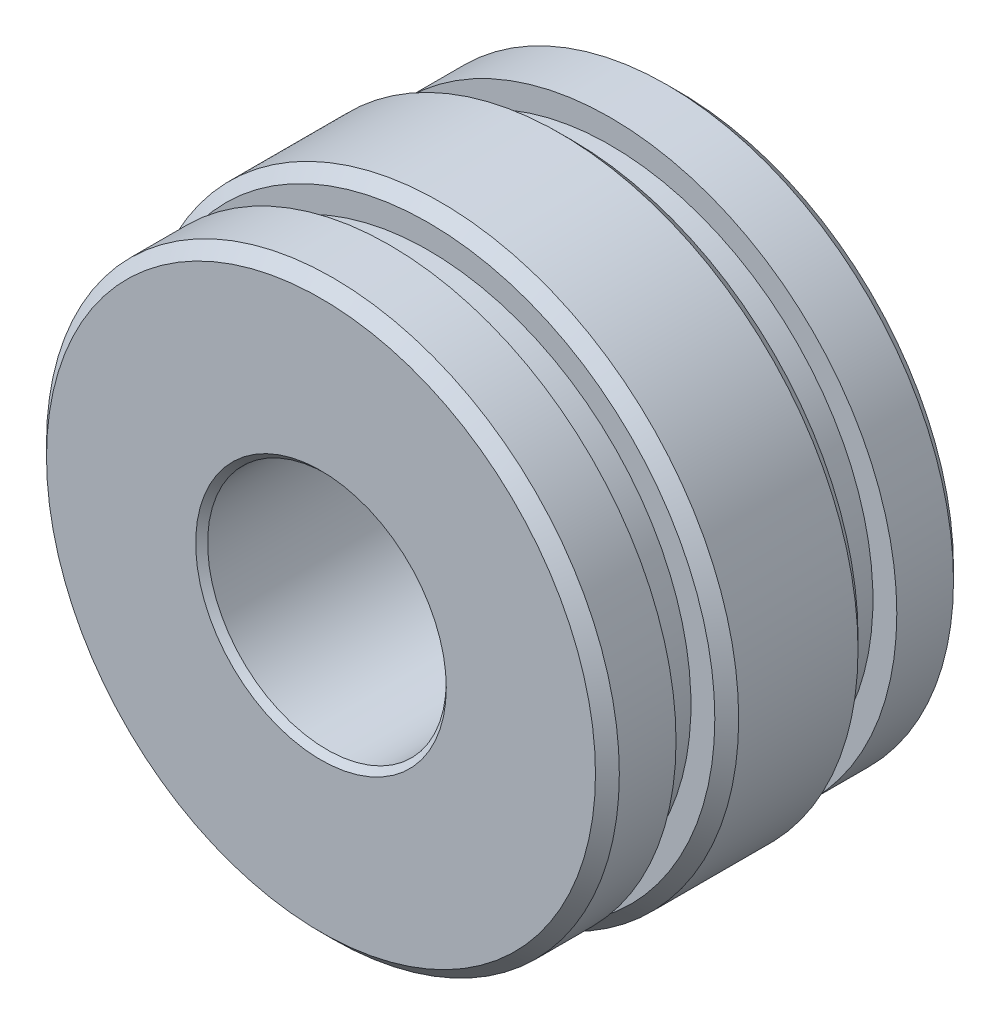
SolidWorks part; units mm, degrees
ref_plane "Front Plane" through (0, 0, 0) normal (0, 0, 1) x (1, 0, 0)
ref_plane "Top Plane" through (0, 0, 0) normal (0, 1, 0) x (1, 0, 0)
ref_plane "Right Plane" through (0, 0, 0) normal (1, 0, 0) x (0, 0, -1)
other "Configuration Table"
sketch "Sketch1" plane through (0, 0, 0) normal (0, 0, 1) x (1, 0, 0)
  circle A0 centre (0, 0) radius 50
  circle A1 centre (0, 0) radius 20
  dimension "D1" = 100
  dimension "D2" = 40
extrude "Boss-Extrude1" add sketch "Sketch1" along normal blind 60
sketch "Sketch2" plane through (0, 0, 0) normal (0, 0, -1) x (-1, 0, 0)
  circle A0 centre (0, 0) radius 44
  circle A1 centre (0, 0) radius 50
  dimension "D1" = 88
extrude "Cut-Extrude1" cut sketch "Sketch2" against normal blind 6.5 from offset 42 offset against normal yes
sketch "Sketch3" plane through (0, 0, 0) normal (0, 0, 1) x (1, 0, 0)
  circle A0 centre (0, 0) radius 44
  circle A1 centre (0, 0) radius 50
  dimension "D1" = 88
extrude "Cut-Extrude2" cut sketch "Sketch3" along normal blind 6.5 from offset 11.5
sketch "Sketch5" plane through (0, 0, 60) normal (0, 0, 1) x (1, 0, 0)
  circle A0 centre (0, 0) radius 48
  circle A1 centre (0, 0) radius 50
  dimension "D1" = 96
extrude "Cut-Extrude3" cut sketch "Sketch5" against normal blind 12
sketch "Sketch6" plane through (0, 0, 0) normal (0, 0, -1) x (-1, 0, 0)
  circle A0 centre (0, 0) radius 50
  circle A1 centre (0, 0) radius 48
  dimension "D1" = 96
  dimension "D2" = 100
extrude "Cut-Extrude4" cut sketch "Sketch6" against normal blind 12
chamfer "Chamfer1" distance 2 angle 45 2 edges at (48, 0, 60) (-48, 0, 0)
chamfer "Chamfer2" distance 1 angle 45 2 edges at (20, 0, 60) (20, 0, 0)
chamfer "Chamfer3" distance 2 angle 45 2 edges at (-50, 0, 42) (50, 0, 18)
